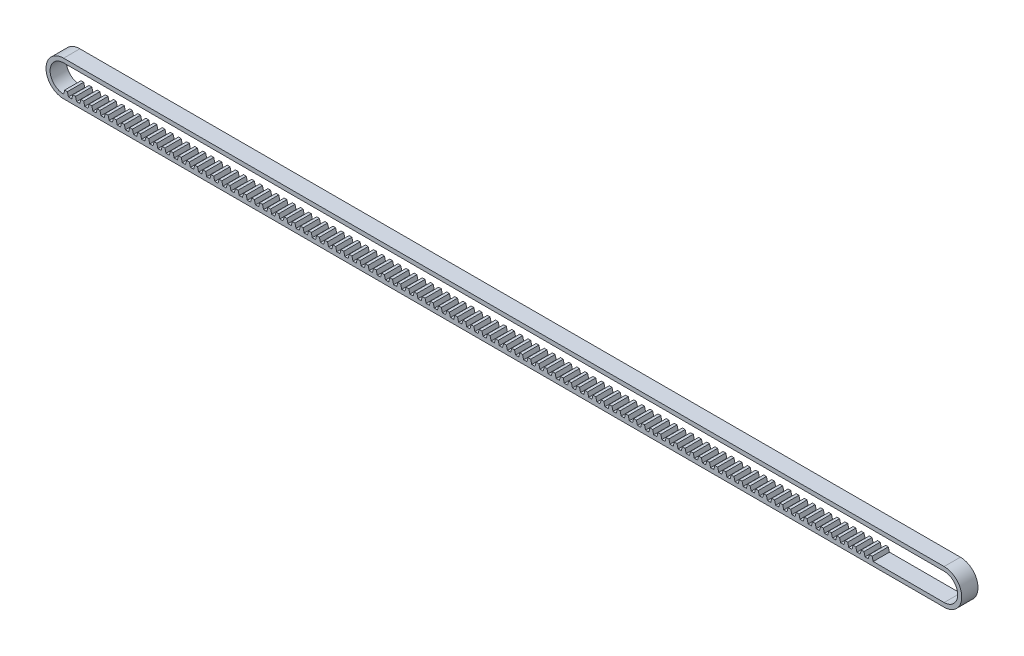
SolidWorks part; units mm, degrees
ref_plane "Front Plane" through (0, 0, 0) normal (0, 0, 1) x (1, 0, 0)
ref_plane "Top Plane" through (0, 0, 0) normal (0, 1, 0) x (1, 0, 0)
ref_plane "Right Plane" through (0, 0, 0) normal (1, 0, 0) x (0, 0, -1)
sketch "Sketch1" plane through (0, 0, 0) normal (0, 0, 1) x (1, 0, 0)
  line L0 (-162.5, -6.5) -> (162.5, -6.5)
  line L1 (-162.5, -5) -> (162.5, -5)
  line L3 (-162.5, 5) -> (162.5, 5)
  line L5 (-162.5, -5) -> (162.5, 5) construction
  line L6 (0, 0) -> (162.5, -5) construction
  line L7 (-162.5, 6.5) -> (162.5, 6.5)
  arc A0 (-162.5, 5) -> (-162.5, -5) centre (-162.5, 0) ccw
  arc A1 (162.5, -5) -> (162.5, 5) centre (162.5, 0) ccw
  arc A2 (162.5, -6.5) -> (162.5, 6.5) centre (162.5, 0) ccw
  arc A3 (-162.5, 6.5) -> (-162.5, -6.5) centre (-162.5, 0) ccw
  arc A5 (-162.1004, 6.4877) -> (-162.1004, -6.4877) centre (-162.5, 0) ccw construction
  arc A6 (-162.1926, 4.9905) -> (-162.1926, -4.9905) centre (-162.5, 0) ccw construction
  arc A7 (162.1004, -6.4877) -> (162.1004, 6.4877) centre (162.5, 0) ccw construction
  arc A8 (162.1926, -4.9905) -> (162.1926, 4.9905) centre (162.5, 0) ccw construction
  point P0 (0, 0)
  dimension "D2" = 10
  dimension "D1" = 325
  dimension "D3" = 1.5
  dimension "D4" = 1.5
extrude "Boss-Extrude1" add sketch "Sketch1" along normal blind 6
sketch "Sketch2" plane through (0, 0, 6) normal (0, 0, 1) x (1, 0, 0)
  line L0 (-162.5, -5) -> (-162.0981, -3.5)
  line L1 (-162.0981, -3.5) -> (-161.0981, -3.5)
  line L2 (-161.0981, -3.5) -> (-160.6962, -5)
  line L4 (-162.5, -5) -> (-160.6962, -5)
  dimension "D1" = 75
  dimension "D2" = 1
  dimension "D3" = 1.5
  dimension "D4" = 75
extrude "Boss-Extrude2" add sketch "Sketch2" against normal blind 6
pattern_linear "LPattern1" count 100 spacing 3 along (1, 0, 0) of "Boss-Extrude2"
